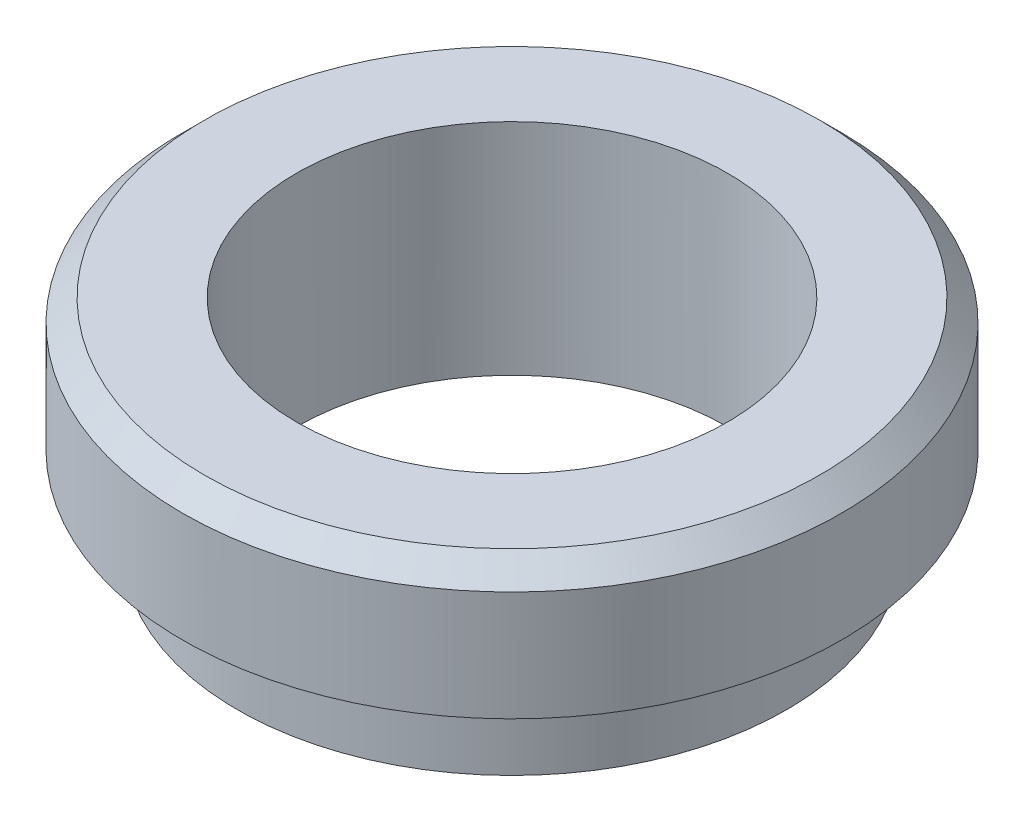
SolidWorks part; units mm, degrees
material "Q235"
ref_plane "Front Plane" through (0, 0, 0) normal (0, 0, 1) x (1, 0, 0)
ref_plane "Top Plane" through (0, 0, 0) normal (0, 1, 0) x (1, 0, 0)
ref_plane "Right Plane" through (0, 0, 0) normal (1, 0, 0) x (0, 0, -1)
sketch "Sketch1" plane through (0, 0, 0) normal (0, 0, 1) x (1, 0, 0)
  line L0 (0, 0) -> (30, 0)
  line L1 (30, 0) -> (30, -12)
  line L2 (30, -12) -> (25, -12)
  line L3 (25, -12) -> (25, -20)
  line L4 (25, -20) -> (0, -20)
  line L5 (0, -20) -> (0, 0)
  dimension "D1" = 25
  dimension "D2" = 30
  dimension "D3" = 8
  dimension "D4" = 12
revolve "Revolve1" add sketch "Sketch1" angle 360 about L5
hole_wizard "G1-1/4 Tapped Hole1" positions "Sketch2" profile "Sketch3" tap size "G1-1/4" standard "GB"
sketch "Sketch2" plane through (0, 0, 0) normal (0, 1, 0) x (1, 0, 0)
  point P0 (0, 0)
sketch "Sketch3" plane through (0, 0, 0) normal (1, 0, 0) x (0, 0, 1)
  line L0 (0, 0) -> (0, 102.5419)
  line L1 (0, 102.5419) -> (19.625, 90.75)
  line L2 (19.625, 90.75) -> (19.625, 0)
  line L5 (19.625, 0) -> (0, 0)
  line L10 (0, 102.5419) -> (-19.625, 90.75) construction
  line L11 (0, -6.35) -> (0, 107.95) construction
  dimension "螺纹孔钻头直径" = 39.25
  dimension "螺纹孔钻头深度" = 90.75
  dimension "导头角度" = 118
cosmetic thread "Hole cosmetic thread1" parameters "D1"=20, "D2"=41.91
chamfer "Chamfer1" distance 2 angle 45 1 edges at (0, 0, -30)
